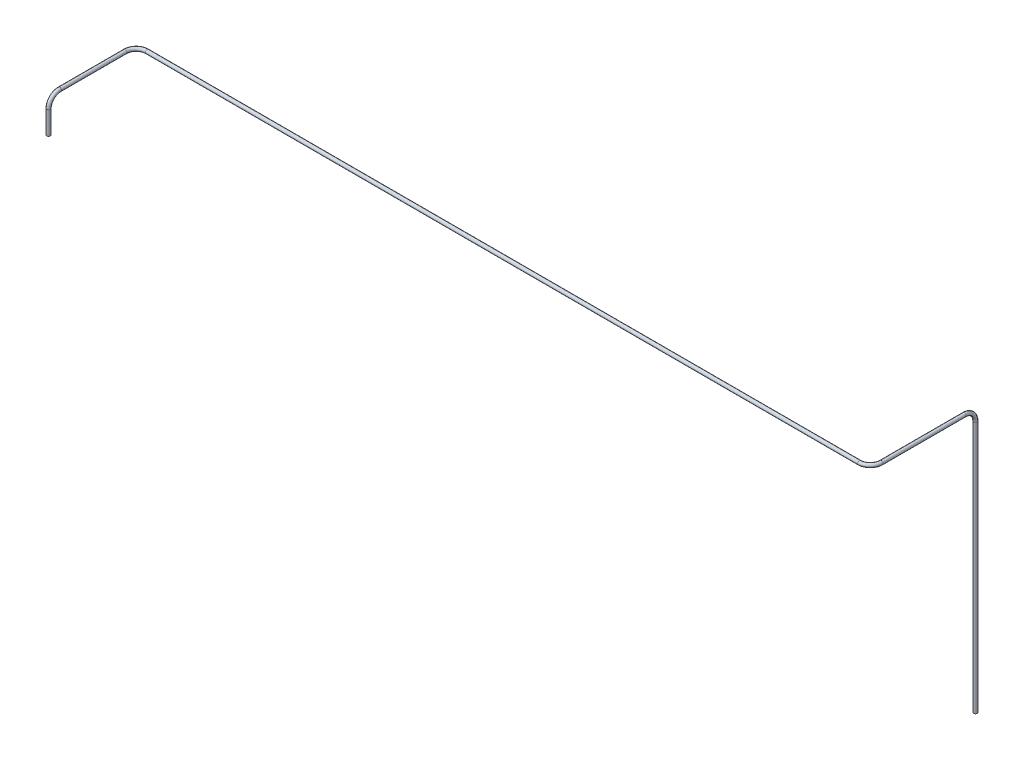
from build123d import *

# Parameters (mm, degrees)
SWEEP_THIN1_PROFILE_R   = 10
SWEEP_THIN1_PROFILE_R_2 = 5


with BuildPart() as part:
    # Sweep-Thin1: sweep along a curve in space
    with BuildLine() as sweep_thin1_path:
        Line((-1700, 2899.052148193, -44.234110711), (-1700, 3024.387350178, -44.234110711))
        ThreePointArc((-1700, 3024.387350178, -44.234110711), (-1700, 3066.813757049, -61.80770384), (-1700, 3084.387350178, -104.234110711))
        Line((-1700, 3084.387350178, -104.234110711), (-1700, 3084.387350178, -461.486974567))
        ThreePointArc((-1700, 3084.387350178, -461.486974567), (-1682.426406871, 3084.387350178, -503.913381439), (-1640, 3084.387350178, -521.486974567))
        Line((-1640, 3084.387350178, -521.486974567), (2240, 3084.387350178, -521.486974567))
        ThreePointArc((2300, 3084.387350178, -581.486974567), (2282.426406871, 3084.387350178, -539.060567696), (2240, 3084.387350178, -521.486974567))
        Line((2300, 3084.387350178, -1034.234110711), (2300, 3084.387350178, -581.486974567))
        ThreePointArc((2300, 3024.387350178, -1094.234110711), (2300, 3066.813757049, -1076.660517582), (2300, 3084.387350178, -1034.234110711))
        Line((2300, 1649.469779319, -1094.234110711), (2300, 3024.387350178, -1094.234110711))
    # Sweep-Thin1 profile (on start of the path) → Sweep-Thin1 (sweep)
    with BuildSketch(Plane(origin=(-1700, 2899.052148193, -44.234110711), x_dir=(0, 0, 1), z_dir=(0, 1, 0))):
        Circle(SWEEP_THIN1_PROFILE_R)
        Circle(SWEEP_THIN1_PROFILE_R_2, mode=Mode.SUBTRACT)
    sweep(path=sweep_thin1_path.line)


solid = part.part
